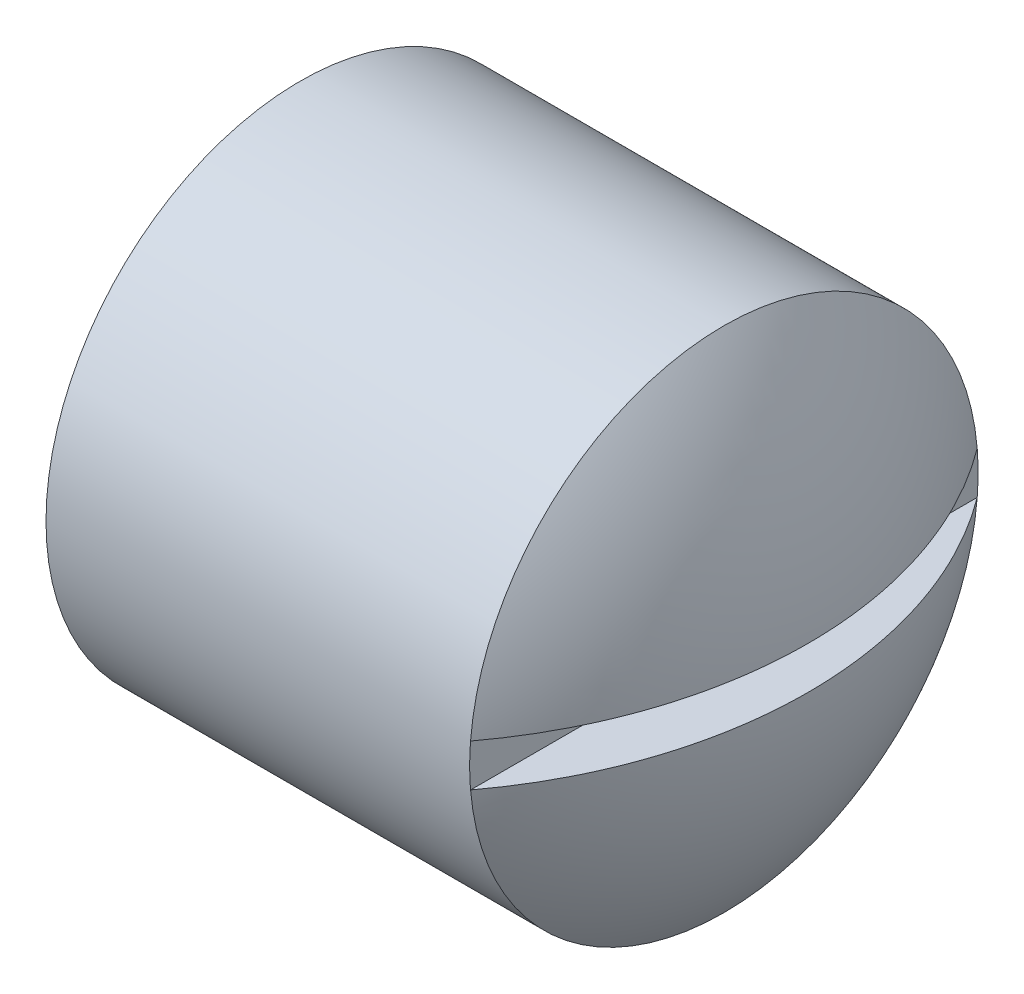
SolidWorks part; units mm, degrees
ref_plane "Front Plane" through (0, 0, 0) normal (0, 0, 1) x (1, 0, 0)
ref_plane "Top Plane" through (0, 0, 0) normal (0, 1, 0) x (1, 0, 0)
ref_plane "Right Plane" through (0, 0, 0) normal (1, 0, 0) x (0, 0, -1)
other "Configuration Table"
sketch "Sketch1" plane through (0, 0, 0) normal (0, 0, 1) x (1, 0, 0)
  line L0 (0, 0) -> (65.1186, 0) construction
  line L1 (0, 0) -> (0, 12)
  line L2 (0, 12) -> (20, 12)
  line L3 (0, 0) -> (24, 0)
  arc A0 (20, 12) -> (24, 0) centre (4, 0) cw
  dimension "D1" = 12
  dimension "D4" = 20
  dimension "D2" = 24
  dimension "D3" = 20
revolve "Revolve1" add sketch "Sketch1" angle 360 about L0
cosmetic thread "Cosmetic Thread1" parameters "D2"=20.752
sketch "Sketch2" plane through (0, 0, 0) normal (0, 0, 1) x (1, 0, 0)
  line L0 (20, 12) -> (20, -12) construction
  line L1 (28, -1) -> (20, -1)
  line L2 (28, -1) -> (28, 1)
  line L3 (28, 1) -> (20, 1)
  line L4 (20, -1) -> (20, 1)
  line L5 (28, -1) -> (20, 1) construction
  line L6 (28, 1) -> (20, -1) construction
  arc A0 (20, -12) -> (20, 12) centre (4, 0) ccw construction
  point P0 (24, 0)
  dimension "D1" = 2
extrude "Cut-Extrude1" cut sketch "Sketch2" against normal through all both and the other way through all
